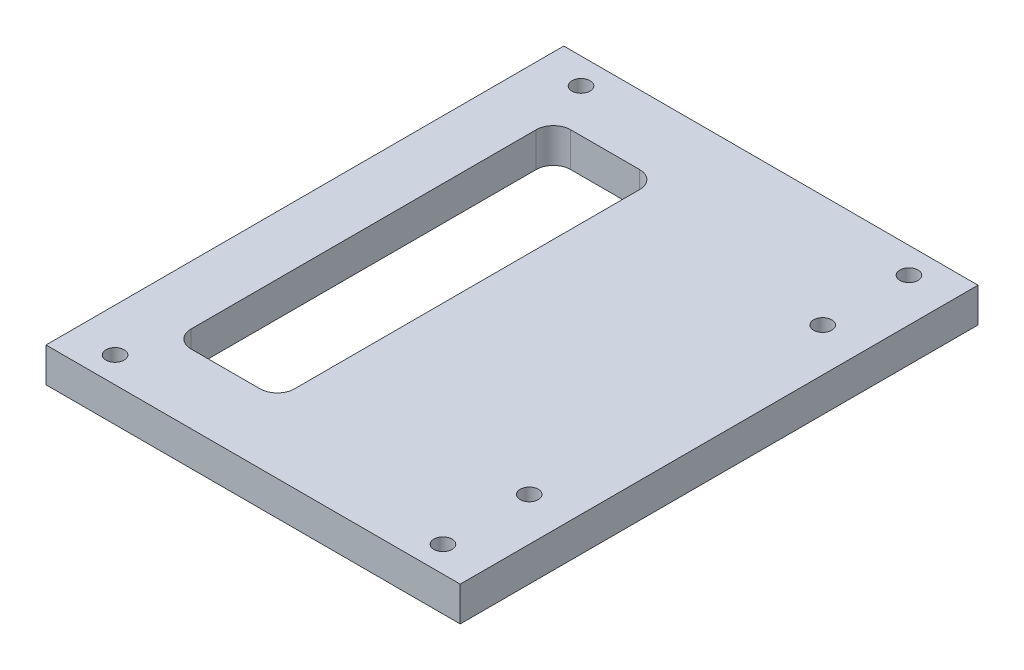
from build123d import *

# Parameters (mm, degrees)
SKETCH1_W           = 480
SKETCH1_H           = 600
BOSS_EXTRUDE1_DEPTH = 40
SKETCH4_W           = 120
SKETCH4_H           = 440
CUT_EXTRUDE3_DEPTH  = 387.264158317
FILLET1_R           = 20
M24_TAPPED_HOLE1_D  = 21


with BuildPart() as part:
    # Sketch1 → Boss-Extrude1 (new body)
    with BuildSketch(Plane(origin=(0, 0, 0), x_dir=(1, 0, 0), z_dir=(0, 1, 0))):
        Rectangle(SKETCH1_W, SKETCH1_H)
    extrude(amount=BOSS_EXTRUDE1_DEPTH)

    # Sketch4 → Cut-Extrude3 (cut, through all)
    with BuildSketch(Plane(origin=(0, 40, 0), x_dir=(1, 0, 0), z_dir=(0, 1, 0))):
        with Locations((-112, 0)):
            Rectangle(SKETCH4_W, SKETCH4_H)
    extrude(amount=-CUT_EXTRUDE3_DEPTH, mode=Mode.SUBTRACT)

    # Fillet1
    fillet1_edges = [part.edges().sort_by_distance(p)[0] for p in [
        (-52, 20, -220),
        (-52, 20, 220),
        (-172, 20, 220),
        (-172, 20, -220),
    ]]
    fillet(fillet1_edges, radius=FILLET1_R)

    # M24 Tapped Hole1 (through all)
    with Locations(Plane(origin=(0, 40, 0), x_dir=(1, 0, 0), z_dir=(0, 1, 0))):
        with Locations((-190, -270), (-190, 270), (190, 270), (190, -270), (190, 170), (190, -170)):
            Hole(M24_TAPPED_HOLE1_D / 2)


solid = part.part
